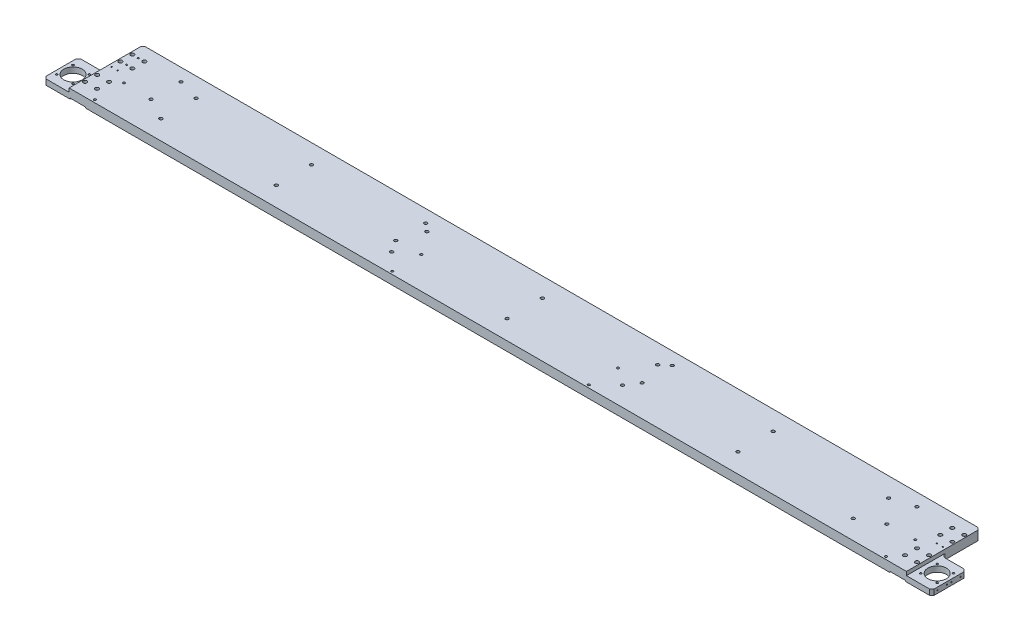
from build123d import *

# Parameters (mm, degrees)
SKETCH_1_W                     = 1924
SKETCH_1_H                     = 160
EXTRUDE_1_DEPTH                = 20
CHAMFER_1_SIZE                 = 5
SKETCH_2_W                     = 55
SKETCH_2_H                     = 8
CUT_EXTRUDE_1_DEPTH            = 976.419909577
SKETCH_3_W                     = 34
SKETCH_3_H                     = 2
CUT_EXTRUDE_3_DEPTH            = 976.419909577
HOLE_WIZARD_M4_1_D             = 4.5
HOLE_WIZARD_M4_1_CBORE_D       = 8
HOLE_WIZARD_M4_1_CBORE_DEPTH   = 14.6
HOLE_WIZARD_M5_1_D             = 4.2
SKETCH_13_R                    = 20
CUT_EXTRUDE_4_DEPTH            = 966.527834917
SKETCH_14_W                    = 55
SKETCH_14_H                    = 85
CUT_EXTRUDE_5_DEPTH            = 966.395255841
CHAMFER_2_SIZE                 = 5
FILLET_1_R                     = 10
HOLE_WIZARD_M6_1_D             = 5
HOLE_WIZARD_M6_1_2_D           = 6.6
HOLE_WIZARD_M6_1_2_CBORE_D     = 11
HOLE_WIZARD_M6_1_2_CBORE_DEPTH = 6.8
HOLE_WIZARD_M8_1_D             = 6.8
CHAMFER_3_SIZE                 = 5
FILLET_2_R                     = 10
HOLE_WIZARD_M3_1_D             = 2.5
HOLE_WIZARD_M3_1_DEPTH         = 7.5
HOLE_WIZARD_M3_1_TIP           = 0.751075774
HOLE_WIZARD_M3_2_AT_2_COUNT    = 2
HOLE_WIZARD_M3_2_AT_2_PITCH    = 50
HOLE_WIZARD_M3_3_AT_2_COUNT    = 2
HOLE_WIZARD_M3_3_AT_2_PITCH    = 13
HOLE_WIZARD_M4_1_2_D           = 3.3
HOLE_WIZARD_M4_1_2_DEPTH       = 10.1
HOLE_WIZARD_M4_1_2_TIP         = 0.991420021


with BuildPart() as part:
    # 草图1 → 凸台-拉伸1 (new body)
    with BuildSketch(Plane(origin=(0, 0, 0), x_dir=(1, 0, 0), z_dir=(0, 1, 0))):
        Rectangle(SKETCH_1_W, SKETCH_1_H)
    extrude(amount=EXTRUDE_1_DEPTH)

    # 倒角1
    chamfer_1_edges = [part.edges().sort_by_distance(p)[0] for p in [
        (962, 10, 80),
        (-962, 10, 80),
        (-962, 10, -80),
        (962, 10, -80),
    ]]
    chamfer(chamfer_1_edges, length=CHAMFER_1_SIZE)

    # 草图2 → 切除-拉伸1 (cut, symmetric)
    with BuildSketch(Plane.XY.offset(80)):
        with Locations((934.5, 16)):
            Rectangle(SKETCH_2_W, SKETCH_2_H)
    cut_extrude_1 = extrude(amount=CUT_EXTRUDE_1_DEPTH, both=True, mode=Mode.SUBTRACT)

    # 镜向1: 切除-拉伸1 across plane
    add(cut_extrude_1.mirror(Plane(origin=(0, 0, 0), x_dir=(0, 0, 1), z_dir=(1, 0, 0))), mode=Mode.SUBTRACT)

    # 草图3 → 切除-拉伸3 (cut, through all)
    with BuildSketch(Plane.XY.offset(80)):
        with Locations((888, 1)):
            Rectangle(SKETCH_3_W, SKETCH_3_H)
    cut_extrude_3 = extrude(amount=-CUT_EXTRUDE_3_DEPTH, mode=Mode.SUBTRACT)

    # Hole Wizard M4 _1 (through all)
    with Locations(Plane(origin=(0, 20, 0), x_dir=(1, 0, 0), z_dir=(0, 1, 0))):
        with Locations((901.042753413, -25.2), (875.042753413, -25.2), (875.042753413, -51.2), (901.042753413, -51.2), (901.042753413, 25.2), (875.042753413, 25.2), (875.042753413, 51.2), (901.042753413, 51.2)):
            hole_wizard_m4_1 = CounterBoreHole(HOLE_WIZARD_M4_1_D / 2, HOLE_WIZARD_M4_1_CBORE_D / 2, HOLE_WIZARD_M4_1_CBORE_DEPTH)

    # M5 螺纹孔1 (through all)
    with Locations(Plane(origin=(0, 12, 0), x_dir=(1, 0, 0), z_dir=(0, 1, 0))):
        with Locations((953.67766953, -24.82233047), (918.32233047, -24.82233047), (953.67766953, -60.17766953), (918.32233047, -60.17766953)):
            hole_wizard_m5_1 = Hole(HOLE_WIZARD_M5_1_D / 2)

    # 草图13 → 切除-拉伸4 (cut, through all)
    with BuildSketch(Plane.XZ):
        with Locations(Location((936, 42.5, 0), (0, 0, 270))):
            Circle(SKETCH_13_R)
    cut_extrude_4 = extrude(amount=-CUT_EXTRUDE_4_DEPTH, mode=Mode.SUBTRACT)

    # 草图14 → 切除-拉伸5 (cut, through all)
    with BuildSketch(Plane(origin=(0, 12, 0), x_dir=(1, 0, 0), z_dir=(0, 1, 0))):
        with Locations((934.5, 37.5)):
            Rectangle(SKETCH_14_W, SKETCH_14_H)
    cut_extrude_5 = extrude(amount=-CUT_EXTRUDE_5_DEPTH, mode=Mode.SUBTRACT)

    # 倒角2
    chamfer_2_edges = [part.edges().sort_by_distance(p)[0] for p in [
        (962, 6, 5),
    ]]
    chamfer(chamfer_2_edges, length=CHAMFER_2_SIZE)

    # 圆角1
    fillet_1_edges = [part.edges().sort_by_distance(p)[0] for p in [
        (907, 6, 5),
    ]]
    fillet(fillet_1_edges, radius=FILLET_1_R)

    # Hole Wizard M6 _1 (through all)
    with Locations(Plane(origin=(0, 20, 0), x_dir=(1, 0, 0), z_dir=(0, 1, 0))):
        with Locations((857, -74), (857, -11), (213, -11), (213, -74)):
            hole_wizard_m6_1 = Hole(HOLE_WIZARD_M6_1_D / 2)

    # Hole Wizard M6 _1 2 (through all)
    with Locations(Plane(origin=(0, 0, 0), x_dir=(-1, 0, 0), z_dir=(0, -1, 0))):
        with Locations((-267, -12.5), (-267, 52.5), (-797, -12.5), (-797, 52.5)):
            hole_wizard_m6_1_2 = CounterBoreHole(HOLE_WIZARD_M6_1_2_D / 2, HOLE_WIZARD_M6_1_2_CBORE_D / 2, HOLE_WIZARD_M6_1_2_CBORE_DEPTH)

    # M8 螺纹孔1 (through all)
    with Locations(Plane(origin=(0, 0, 0), x_dir=(-1, 0, 0), z_dir=(0, -1, 0))):
        with Locations((750, 38.2), (750, -38.2), (500, 38.2), (500, -38.2), (250, 38.2), (250, -38.2), (0, 38.2), (0, -38.2), (-250, 38.2), (-250, -38.2), (-500, 38.2), (-500, -38.2), (-750, 38.2), (-750, -38.2)):
            Hole(HOLE_WIZARD_M8_1_D / 2)

    # 镜向4: 切除-拉伸3, Hole Wizard M4 _1, M5 螺纹孔1, 切除-拉伸4, 切除-拉伸5, Hole Wizard M6 _1, Hole Wizard M6 _1 2 across plane
    add(cut_extrude_3.mirror(Plane(origin=(0, 0, 0), x_dir=(0, 0, 1), z_dir=(1, 0, 0))), mode=Mode.SUBTRACT)
    add(hole_wizard_m4_1.mirror(Plane(origin=(0, 0, 0), x_dir=(0, 0, 1), z_dir=(1, 0, 0))), mode=Mode.SUBTRACT)
    add(hole_wizard_m5_1.mirror(Plane(origin=(0, 0, 0), x_dir=(0, 0, 1), z_dir=(1, 0, 0))), mode=Mode.SUBTRACT)
    add(cut_extrude_4.mirror(Plane(origin=(0, 0, 0), x_dir=(0, 0, 1), z_dir=(1, 0, 0))), mode=Mode.SUBTRACT)
    add(cut_extrude_5.mirror(Plane(origin=(0, 0, 0), x_dir=(0, 0, 1), z_dir=(1, 0, 0))), mode=Mode.SUBTRACT)
    add(hole_wizard_m6_1.mirror(Plane(origin=(0, 0, 0), x_dir=(0, 0, 1), z_dir=(1, 0, 0))), mode=Mode.SUBTRACT)
    add(hole_wizard_m6_1_2.mirror(Plane(origin=(0, 0, 0), x_dir=(0, 0, 1), z_dir=(1, 0, 0))), mode=Mode.SUBTRACT)

    # 倒角3
    chamfer_3_edges = [part.edges().sort_by_distance(p)[0] for p in [
        (907, 10, -80),
        (-962, 6, 5),
        (-907, 10, -80),
    ]]
    chamfer(chamfer_3_edges, length=CHAMFER_3_SIZE)

    # 圆角2
    fillet_2_edges = [part.edges().sort_by_distance(p)[0] for p in [
        (-907, 6, 5),
    ]]
    fillet(fillet_2_edges, radius=FILLET_2_R)

    # M3 螺纹孔1
    with Locations(Plane(origin=(962, 0, 0), x_dir=(0, 0, -1), z_dir=(1, 0, 0))):
        with Locations((-47.5, 6), (-37.5, 6)):
            Hole(HOLE_WIZARD_M3_1_D / 2, depth=HOLE_WIZARD_M3_1_DEPTH)
            with Locations((0, 0, -(HOLE_WIZARD_M3_1_DEPTH + HOLE_WIZARD_M3_1_TIP / 2))):  # 118° drill point
                Cone(0, HOLE_WIZARD_M3_1_D / 2, HOLE_WIZARD_M3_1_TIP, mode=Mode.SUBTRACT)

    # 草图28 → M3 螺纹孔2 (revolve, cut)
    with BuildSketch(Plane(origin=(962, 6, 67.5), x_dir=(0, 0, -1), z_dir=(0, 1, 0))):
        Polygon((0, 0), (0, 8.251075774), (1.25, 7.5), (1.25, 0), align=None)
    hole_wizard_m3_2 = revolve(axis=Axis((968.35, 6, 67.5), (-1, 0, 0)), mode=Mode.SUBTRACT)

    # M3 螺纹孔2 at 2: M3 螺纹孔2 ×2
    with Locations(*[(0, 0, -i * HOLE_WIZARD_M3_2_AT_2_PITCH) for i in range(1, HOLE_WIZARD_M3_2_AT_2_COUNT)]):
        add(hole_wizard_m3_2, mode=Mode.SUBTRACT)

    # 草图31 → M3 螺纹孔3 (revolve, cut)
    with BuildSketch(Plane(origin=(887.5, 20, -5.5), x_dir=(0, 0, 1), z_dir=(1, 0, 0))):
        Polygon((0, 0), (0, 8.251075774), (1.25, 7.5), (1.25, 0), align=None)
    hole_wizard_m3_3 = revolve(axis=Axis((887.5, 26.35, -5.5), (0, -1, 0)), mode=Mode.SUBTRACT)

    # M3 螺纹孔3 at 2: M3 螺纹孔3 ×2
    with Locations(*[(i * HOLE_WIZARD_M3_3_AT_2_PITCH, 0, 0) for i in range(1, HOLE_WIZARD_M3_3_AT_2_COUNT)]):
        add(hole_wizard_m3_3, mode=Mode.SUBTRACT)

    # 镜向5: M3 螺纹孔2, M3 螺纹孔3 across plane
    add(hole_wizard_m3_2.mirror(Plane(origin=(0, 0, 0), x_dir=(0, 0, 1), z_dir=(1, 0, 0))), mode=Mode.SUBTRACT)
    add(hole_wizard_m3_3.mirror(Plane(origin=(0, 0, 0), x_dir=(0, 0, 1), z_dir=(1, 0, 0))), mode=Mode.SUBTRACT)

    # 镜向5 copy 1 sketch → 镜向5 copy 1 (revolve, cut)
    with BuildSketch(Plane(origin=(-962, 6, 17.5), x_dir=(0, 0, -1), z_dir=(0, 1, 0))):
        Polygon((0, 0), (0, -8.251075774), (1.25, -7.5), (1.25, 0), align=None)
    revolve(axis=Axis((-968.35, 6, 17.5), (-1, 0, 0)), mode=Mode.SUBTRACT)

    # 镜向5 copy 2 sketch → 镜向5 copy 2 (revolve, cut)
    with BuildSketch(Plane(origin=(-900.5, 20, -5.5), x_dir=(0, 0, 1), z_dir=(-1, 0, 0))):
        Polygon((0, 0), (0, -8.251075774), (1.25, -7.5), (1.25, 0), align=None)
    revolve(axis=Axis((-900.5, 26.35, -5.5), (0, 1, 0)), mode=Mode.SUBTRACT)

    # Hole Wizard M4 _1 2
    with Locations(Plane(origin=(0, 20, 0), x_dir=(1, 0, 0), z_dir=(0, 1, 0))):
        with Locations((-888, 50.7), (-888, 25.7)):
            Hole(HOLE_WIZARD_M4_1_2_D / 2, depth=HOLE_WIZARD_M4_1_2_DEPTH)
            with Locations((0, 0, -(HOLE_WIZARD_M4_1_2_DEPTH + HOLE_WIZARD_M4_1_2_TIP / 2))):  # 118° drill point
                Cone(0, HOLE_WIZARD_M4_1_2_D / 2, HOLE_WIZARD_M4_1_2_TIP, mode=Mode.SUBTRACT)


solid = part.part
